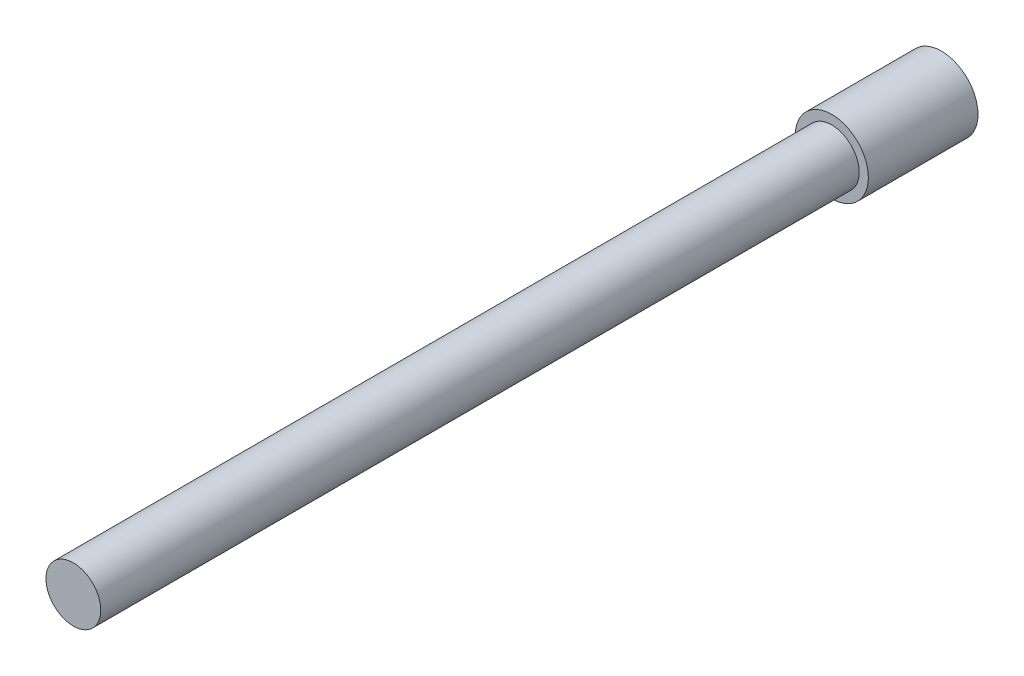
SolidWorks part; units mm, degrees
material "AISI 304"
ref_plane "前视基准面" through (0, 0, 0) normal (0, 0, 1) x (1, 0, 0)
ref_plane "上视基准面" through (0, 0, 0) normal (0, 1, 0) x (1, 0, 0)
ref_plane "右视基准面" through (0, 0, 0) normal (1, 0, 0) x (0, 0, -1)
sketch "草图1" plane through (0, 0, 0) normal (0, 0, 1) x (1, 0, 0)
  circle A0 centre (0, 0) radius 4
  dimension "D1" = 8
extrude "凸台-拉伸1" add sketch "草图1" along normal blind 95
sketch "草图2" plane through (0, 0, 95) normal (0, 0, 1) x (1, 0, 0)
  circle A0 centre (0, 0) radius 4
  circle A1 centre (0, 0) radius 3
  dimension "D1" = 6
extrude "切除-拉伸1" cut sketch "草图2" against normal blind 83
